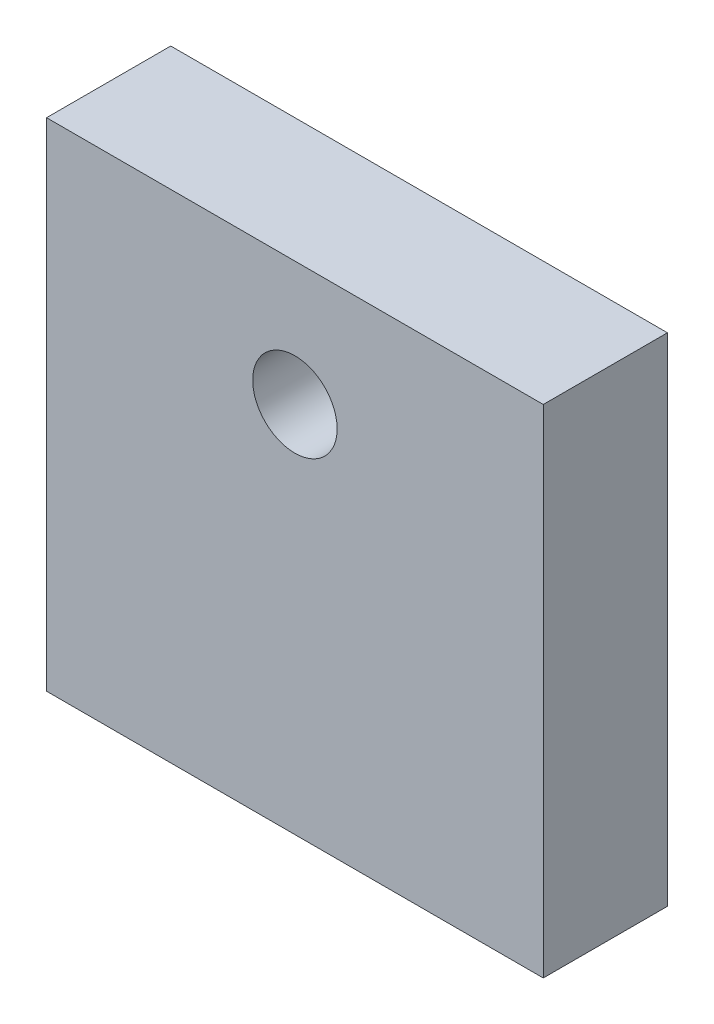
from build123d import *

# Parameters (mm, degrees)
SKETCH_1_W         = 40
SKETCH_1_H         = 40
EXTRUDE_1_DEPTH    = 5
HOLE_WIZARD_M8_1_D = 6.8


with BuildPart() as part:
    # 草图1 → 凸台-拉伸1 (new, symmetric)
    with BuildSketch(Plane.XY):
        Rectangle(SKETCH_1_W, SKETCH_1_H)
    extrude(amount=EXTRUDE_1_DEPTH, both=True)

    # M8 螺纹孔1 (through all)
    with Locations(Plane.XY.offset(5)):
        with Locations((0, 10)):
            Hole(HOLE_WIZARD_M8_1_D / 2)


solid = part.part
